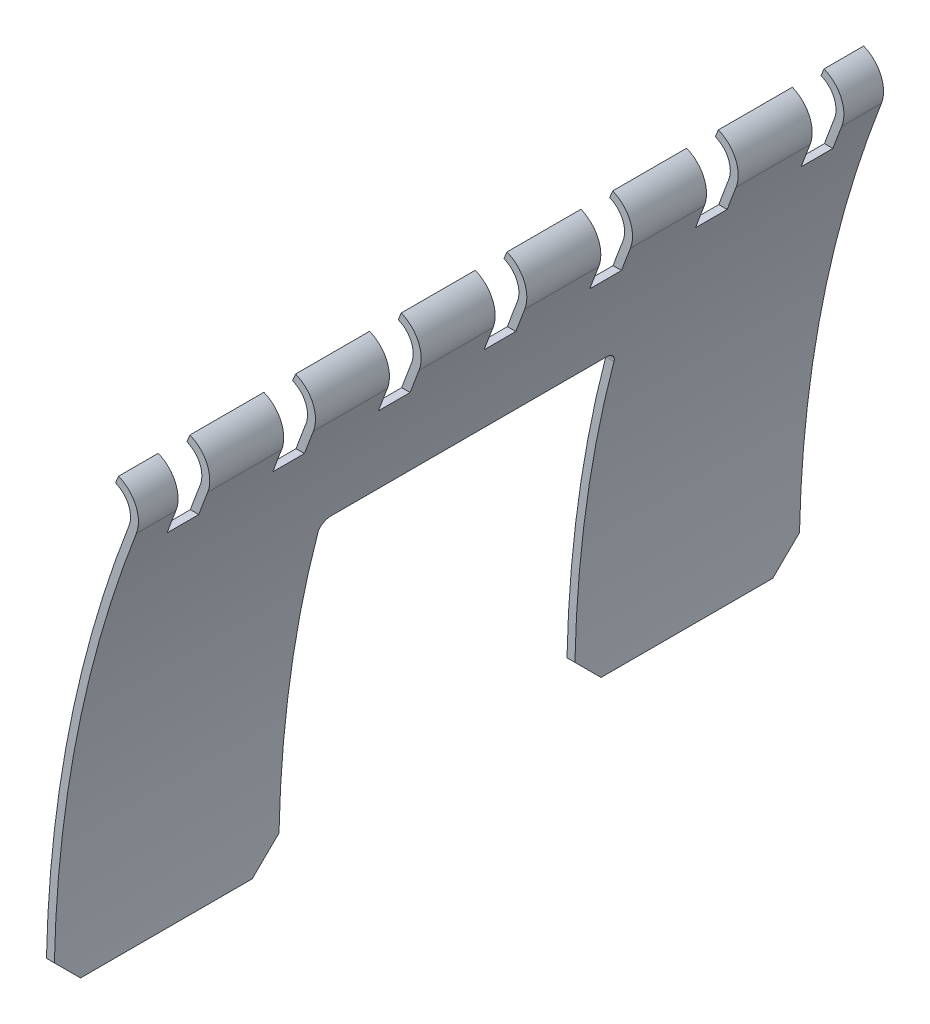
from build123d import *

# Parameters (mm, degrees)
BOSS_EXTRUDE1_DEPTH = 70.5
SKETCH2_W           = 62.190757718
SKETCH2_H           = 82.229138737
CUT_EXTRUDE1_DEPTH  = 28
FILLET1_R           = 2
CHAMFER2_SIZE       = 5
SKETCH3_W           = 6
SKETCH3_H           = 12.2
CUT_EXTRUDE2_DEPTH  = 259.304651789


with BuildPart() as part:
    # Sketch1 → Boss-Extrude1 (new, symmetric)
    with BuildSketch(Plane.XY):
        with BuildLine():
            Line((-229.8, 0), (-231.3, 0))
            ThreePointArc((-231.3, 0), (-227.352946258, 42.547947397), (-215.646495221, 83.64376306))
            ThreePointArc((-215.646495221, 83.64376306), (-215.716016682, 87.067362872), (-218.174682858, 89.450811957))
            ThreePointArc((-218.174682858, 89.450811957), (-217.889049095, 90.144341388), (-217.601210761, 90.836958751))
            ThreePointArc((-217.601210761, 90.836958751), (-214.336902597, 87.65737358), (-214.248009519, 83.101326205))
            ThreePointArc((-214.248009519, 83.101326205), (-225.878543235, 42.272020371), (-229.8, 0))
        make_face()
    extrude(amount=BOSS_EXTRUDE1_DEPTH, both=True)

    # Sketch2 → Cut-Extrude1 (cut, symmetric)
    with BuildSketch(Plane.XY):
        with Locations((-225.789861071, 18.885430632)):
            Rectangle(SKETCH2_W, SKETCH2_H)
    extrude(amount=CUT_EXTRUDE1_DEPTH, both=True, mode=Mode.SUBTRACT)

    # Fillet1
    fillet1_edges = [part.edges().sort_by_distance(p)[0] for p in [
        (-222.605619054, 60, -28),
        (-222.605619054, 60, 28),
    ]]
    fillet(fillet1_edges, radius=FILLET1_R)

    # Chamfer2
    chamfer2_edges = [part.edges().sort_by_distance(p)[0] for p in [
        (-230.55, 0, 70.5),
        (-230.55, 0, 28),
        (-230.55, 0, -28),
        (-230.55, 0, -70.5),
    ]]
    chamfer(chamfer2_edges, length=CHAMFER2_SIZE)

    # Sketch3 → Cut-Extrude2 (cut, through all)
    with BuildSketch(Plane(origin=(0, 0, 0), x_dir=(0, 0, -1), z_dir=(1, 0, 0))):
        with Locations((60, 84.736958751)):
            Rectangle(SKETCH3_W, SKETCH3_H)
        with Locations((40, 84.736958751)):
            Rectangle(SKETCH3_W, SKETCH3_H)
        with Locations((20, 84.736958751)):
            Rectangle(SKETCH3_W, SKETCH3_H)
        with Locations((0, 84.736958751)):
            Rectangle(SKETCH3_W, SKETCH3_H)
        with Locations((-20, 84.736958751)):
            Rectangle(SKETCH3_W, SKETCH3_H)
        with Locations((-40, 84.736958751)):
            Rectangle(SKETCH3_W, SKETCH3_H)
        with Locations((-60, 84.736958751)):
            Rectangle(SKETCH3_W, SKETCH3_H)
    extrude(amount=-CUT_EXTRUDE2_DEPTH, mode=Mode.SUBTRACT)


solid = part.part
